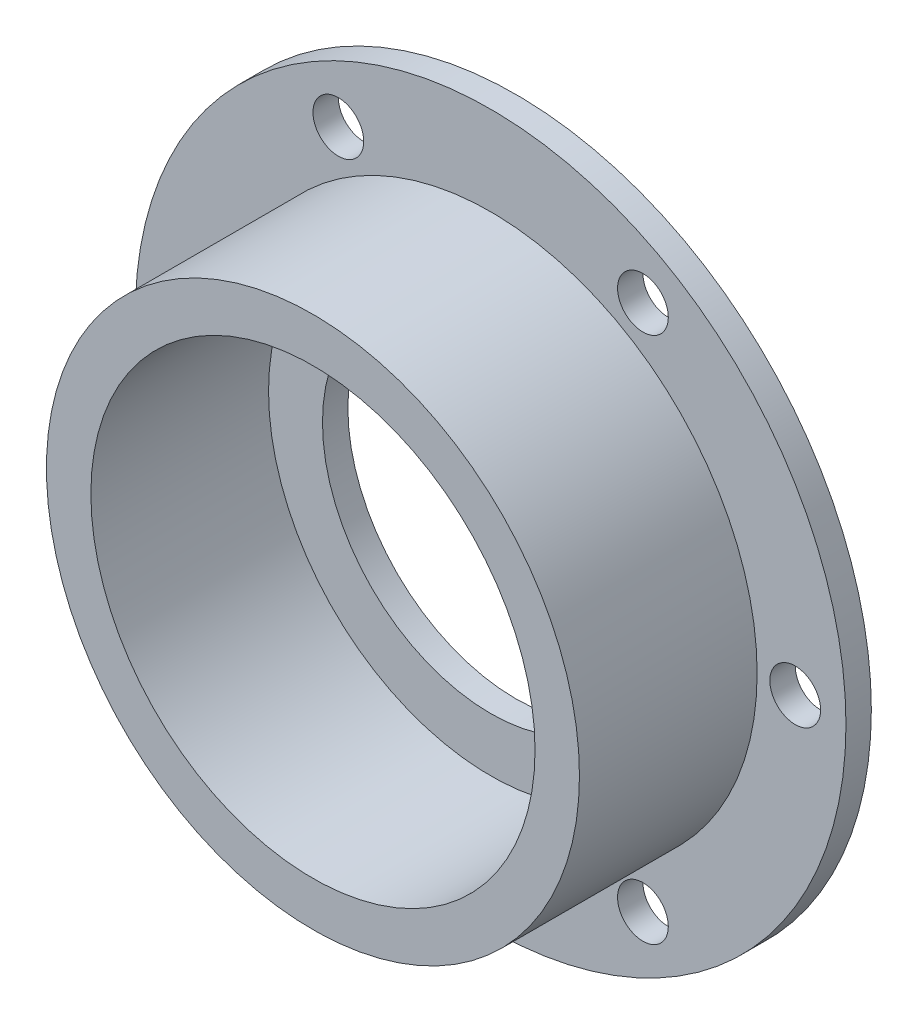
from build123d import *

# Parameters (mm, degrees)
SKETCH_1_R          = 280
EXTRUDE_1_DEPTH     = 20
SKETCH_2_R          = 210
EXTRUDE_2_DEPTH     = 160
SKETCH_3_R          = 175
CUT_EXTRUDE_1_DEPTH = 140
SKETCH_4_R          = 20
CUT_EXTRUDE_3_DEPTH = 20
SKETCH_5_R          = 132.5
CUT_EXTRUDE_4_DEPTH = 20


with BuildPart() as part:
    # 草图1 → 凸台-拉伸1 (new body)
    with BuildSketch(Plane.XY):
        Circle(SKETCH_1_R)
    extrude(amount=EXTRUDE_1_DEPTH)

    # 草图2 → 凸台-拉伸2 (add)
    with BuildSketch(Plane.XY):
        Circle(SKETCH_2_R)
    extrude(amount=EXTRUDE_2_DEPTH)

    # 草图3 → 切除-拉伸1 (cut)
    with BuildSketch(Plane.XY.offset(160)):
        Circle(SKETCH_3_R)
    extrude(amount=-CUT_EXTRUDE_1_DEPTH, mode=Mode.SUBTRACT)

    # 草图4 → 切除-拉伸3 (cut)
    with BuildSketch(Plane.XY):
        with Locations((240, 0)):
            Circle(SKETCH_4_R)
        with Locations((-240, 0)):
            Circle(SKETCH_4_R)
        with Locations((-120, 207.846096908)):
            Circle(SKETCH_4_R)
        with Locations((120, 207.846096908)):
            Circle(SKETCH_4_R)
        with Locations((-120, -207.846096908)):
            Circle(SKETCH_4_R)
        with Locations((120, -207.846096908)):
            Circle(SKETCH_4_R)
    extrude(amount=CUT_EXTRUDE_3_DEPTH, mode=Mode.SUBTRACT)

    # 草图5 → 切除-拉伸4 (cut)
    with BuildSketch(Plane.XY):
        Circle(SKETCH_5_R)
    extrude(amount=CUT_EXTRUDE_4_DEPTH, mode=Mode.SUBTRACT)


solid = part.part
